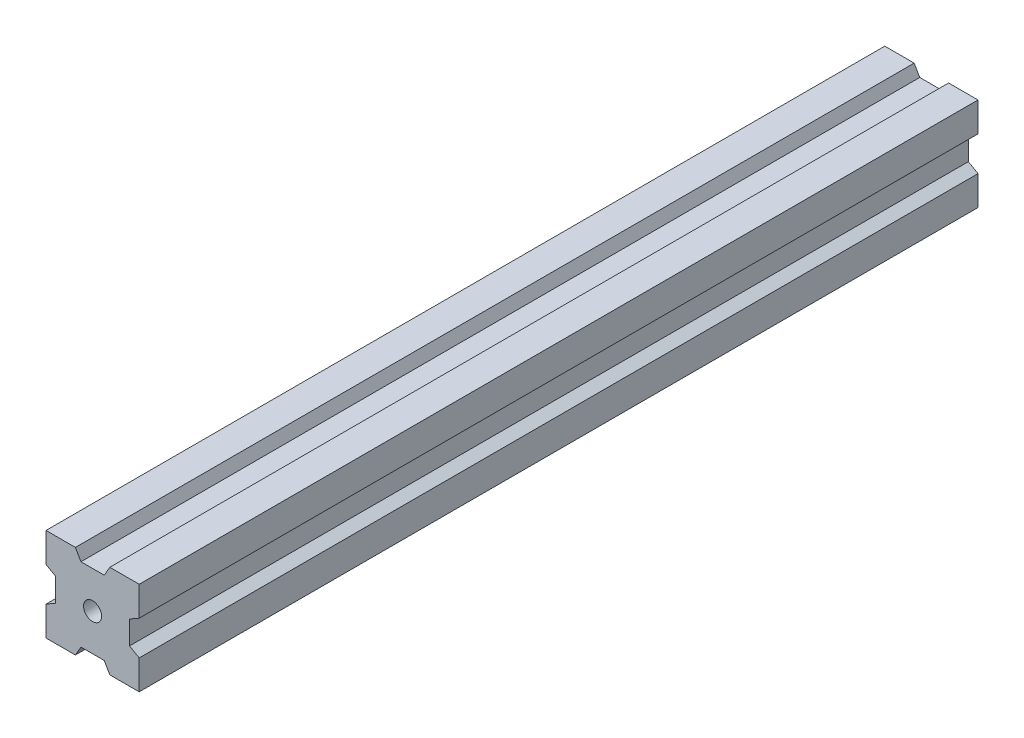
SolidWorks part; units mm, degrees
ref_plane "前视基准面" through (0, 0, 0) normal (0, 0, 1) x (1, 0, 0)
ref_plane "上视基准面" through (0, 0, 0) normal (0, 1, 0) x (1, 0, 0)
ref_plane "右视基准面" through (0, 0, 0) normal (1, 0, 0) x (0, 0, -1)
sketch "草图1" plane through (0, 0, 0) normal (0, 0, 1) x (1, 0, 0)
  line L1 (10, -10) -> (-10, -10)
  line L2 (10, -10) -> (10, 10)
  line L3 (10, 10) -> (-10, 10)
  line L4 (-10, -10) -> (-10, 10)
  line L5 (10, -10) -> (-10, 10) construction
  line L6 (10, 10) -> (-10, -10) construction
  circle A0 centre (0, 0) radius 1.9444
  point P0 (0, 0)
  dimension "D1" = 20
extrude "凸台-拉伸1" add sketch "草图1" along normal mid plane 180
sketch "草图2" plane through (0, 0, 90) normal (0, 0, 1) x (1, 0, 0)
  line L0 (-3.6944, 10) -> (-2.5, 7.9312)
  line L1 (10, 10) -> (-10, 10) construction
  line L2 (-2.5, 7.9312) -> (2.5, 7.9312)
  line L3 (2.5, 7.9312) -> (3.6944, 10)
  line L4 (0, 10) -> (0, 7.9312) construction
  line L5 (-3.6944, 10) -> (3.6944, 10) construction
  dimension "D1" = 5
  dimension "D2" = 60
extrude "切除-拉伸1" cut sketch "草图2" against normal through all and the other way through all
pattern_circular "阵列(圆周)1" count 4 over 360 about axis through (0, 0, 90) along (0, 0, -1) of "切除-拉伸1"
